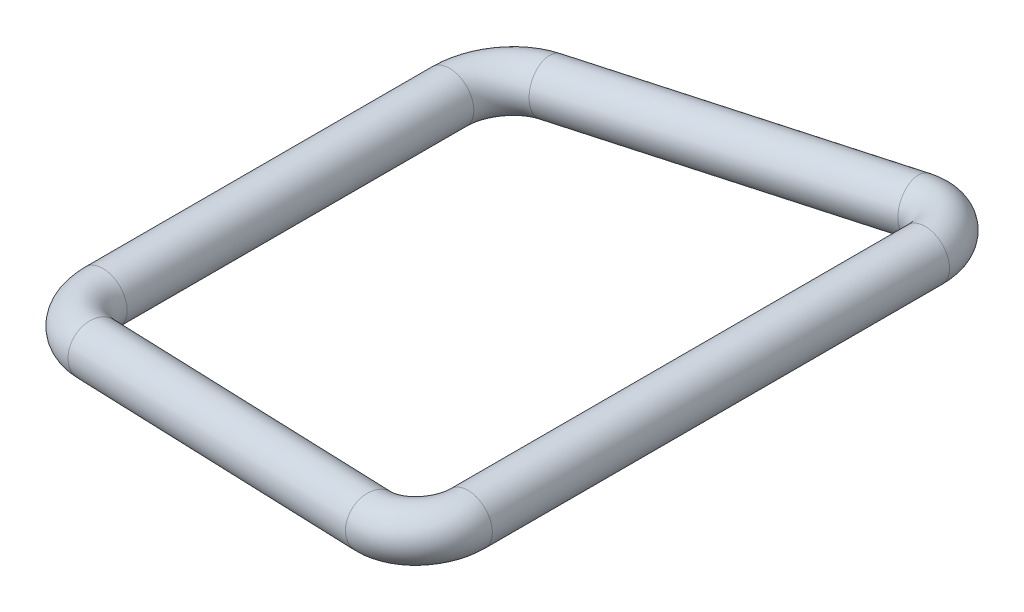
from build123d import *

# Parameters (mm, degrees)
BOSS_EXTRUDE1_DEPTH      = 9.4
BOSS_EXTRUDE1_DEPTH_BACK = 9.4
SKETCH1_R                = 1
SKETCH2_R                = 1
REVOLVE1_ANGLE           = 98
SKETCH3_R                = 1
BOSS_EXTRUDE2_DEPTH      = 13.5
SKETCH5_R                = 1
REVOLVE2_ANGLE           = 98
SKETCH6_R                = 1
BOSS_EXTRUDE3_DEPTH      = 13.5
SKETCH7_R                = 1
REVOLVE3_ANGLE           = 82
SKETCH8_R                = 1
REVOLVE4_ANGLE           = 82
BOSS_EXTRUDE4_DEPTH      = 7.128
BOSS_EXTRUDE4_DEPTH_BACK = 7.128
SKETCH4_R                = 1


with BuildPart() as part:
    # Sketch1 → Boss-Extrude1 (new, two sides: drawn at the far end of the back side and taken through both)
    with BuildSketch(Plane.XY.offset(-BOSS_EXTRUDE1_DEPTH_BACK)):
        Circle(SKETCH1_R)
    extrude(amount=BOSS_EXTRUDE1_DEPTH + BOSS_EXTRUDE1_DEPTH_BACK)

    # Sketch2 → Revolve1 (revolve)
    with BuildSketch(Plane.XY.offset(-9.4)):
        with Locations(Location((0, 0, 0), (0, 0, 6.2))):
            Circle(SKETCH2_R)
    revolve(axis=Axis((-1.634001289, -1.988301928, -9.4), (-0.10799935570602286, 0.9941509639723154, 0)), revolution_arc=REVOLVE1_ANGLE)

    # Sketch3 → Boss-Extrude2 (add)
    with BuildSketch(Plane(origin=(-0.505088704, -0.054870192, 0.071403228), x_dir=(0.13835907247846538, 0.015030605235296325, 0.9902680687415704), z_dir=(-0.9844759551304353, -0.10694831340033709, 0.1391731009600654))):
        with Locations(Location((-11.403663414, 0, 0), (0, 0, 180))):
            Circle(SKETCH3_R)
    extrude(amount=BOSS_EXTRUDE2_DEPTH)

    # Sketch5 → Revolve2 (revolve)
    with BuildSketch(Plane.XY.offset(9.4)):
        with Locations(Location((0, 0, 0), (0, 0, 6.2))):
            Circle(SKETCH5_R)
    revolve(axis=Axis((-1.634001289, -1.988301928, 9.4), (0.10799935570602286, -0.9941509639723154, 0)), revolution_arc=REVOLVE2_ANGLE)

    # Sketch6 → Boss-Extrude3 (add)
    with BuildSketch(Plane(origin=(-0.505088704, -0.054870192, -0.071403228), x_dir=(-0.13835907247846538, -0.015030605235296325, 0.9902680687415704), z_dir=(-0.9844759551304353, -0.10694831340033709, -0.1391731009600654))):
        with Locations((11.403663414, 0)):
            Circle(SKETCH6_R)
    extrude(amount=BOSS_EXTRUDE3_DEPTH)

    # Sketch7 → Revolve3 (revolve)
    with BuildSketch(Plane(origin=(-13.795514099, -1.498672423, 1.950240091), x_dir=(0.13835907247846538, 0.015030605235296325, 0.9902680687415704), z_dir=(-0.9844759551304353, -0.10694831340033709, 0.1391731009600654))):
        with Locations(Location((-11.403663414, 0, 0), (0, 0, 180))):
            Circle(SKETCH7_R)
    revolve(axis=Axis((-20.490038802, 48.312670109, -7.127372755), (-0.10799935570602279, 0.9941509639723154, 0)), revolution_arc=REVOLVE3_ANGLE)

    # Sketch8 → Revolve4 (revolve)
    with BuildSketch(Plane(origin=(-13.795514099, -1.498672423, -1.950240091), x_dir=(-0.13835907247846538, -0.015030605235296325, 0.9902680687415704), z_dir=(-0.9844759551304353, -0.10694831340033709, -0.1391731009600654))):
        with Locations((11.403663414, 0)):
            Circle(SKETCH8_R)
    revolve(axis=Axis((-9.690103231, -51.102426288, 7.127372755), (0.10799935570602279, -0.9941509639723154, 0)), revolution_arc=REVOLVE4_ANGLE)

    # Sketch4 → Boss-Extrude4 (add, two sides: drawn at the far end of the back side and taken through both)
    with BuildSketch(Plane.XY.offset(-BOSS_EXTRUDE4_DEPTH_BACK)):
        with Locations(Location((-17.287589358, -1.878033196, 0), (0, 0, 186.2))):
            Circle(SKETCH4_R)
    extrude(amount=BOSS_EXTRUDE4_DEPTH + BOSS_EXTRUDE4_DEPTH_BACK)


solid = part.part
